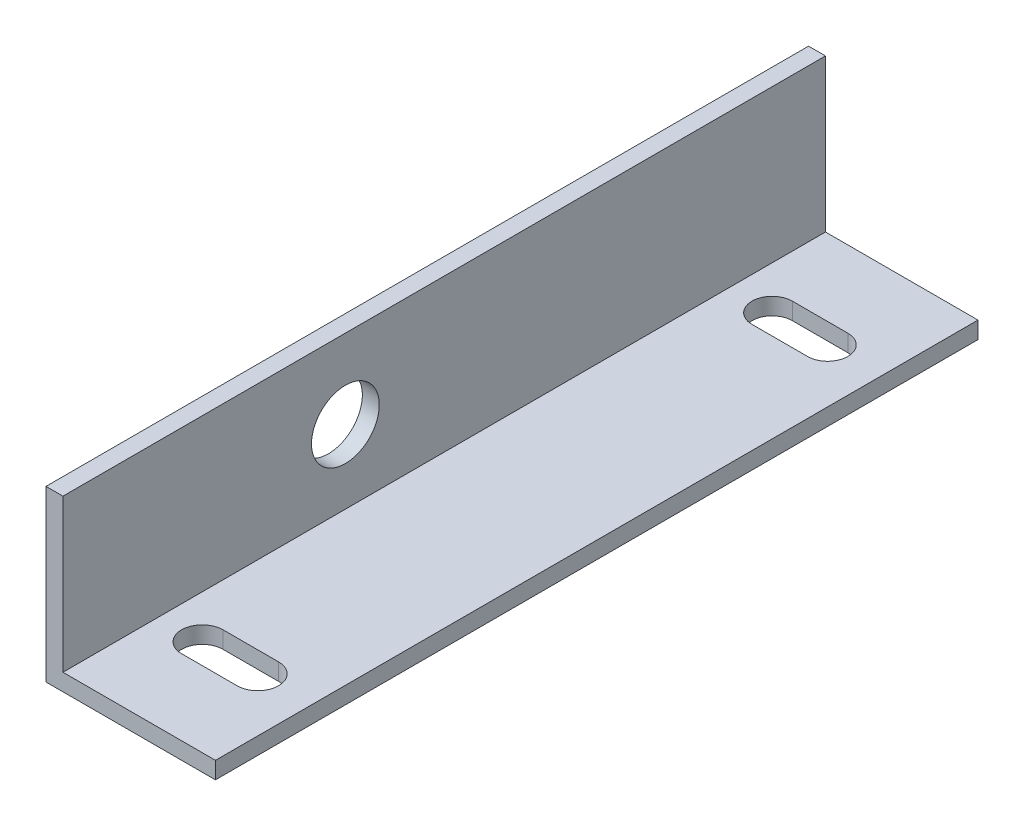
SolidWorks part; units mm, degrees
ref_plane "Front Plane" through (0, 0, 0) normal (0, 0, 1) x (1, 0, 0)
ref_plane "Top Plane" through (0, 0, 0) normal (0, 1, 0) x (1, 0, 0)
ref_plane "Right Plane" through (0, 0, 0) normal (1, 0, 0) x (0, 0, -1)
sketch "Sketch1" plane through (0, 0, 0) normal (0, 0, 1) x (1, 0, 0)
  line L0 (0, 0) -> (0, 30)
  line L1 (0, 0) -> (30, 0)
  line L2 (3, 3) -> (30, 3)
  line L3 (3, 3) -> (3, 30)
  line L4 (0, 30) -> (3, 30)
  line L5 (30, 3) -> (30, 0)
  dimension "D1" = 30
  dimension "D2" = 30
  dimension "D3" = 3
extrude "Boss-Extrude1" add sketch "Sketch1" along normal blind 135
sketch "Sketch2" plane through (0, 3, 0) normal (0, 1, 0) x (1, 0, 0)
  line L0 (10.659, -17.1008) -> (20.4946, -17.1008) construction
  line L1 (10.659, -13.5319) -> (20.4946, -13.5319)
  line L2 (10.659, -20.6697) -> (20.4946, -20.6697)
  line L3 (10.659, -117.9846) -> (20.4946, -117.9846) construction
  line L4 (10.659, -114.3178) -> (20.4946, -114.3178)
  line L5 (10.659, -121.6515) -> (20.4946, -121.6515)
  arc A0 (10.659, -13.5319) -> (10.659, -20.6697) centre (10.659, -17.1008) ccw
  arc A1 (20.4946, -20.6697) -> (20.4946, -13.5319) centre (20.4946, -17.1008) ccw
  arc A2 (10.659, -114.3178) -> (10.659, -121.6515) centre (10.659, -117.9846) ccw
  arc A3 (20.4946, -121.6515) -> (20.4946, -114.3178) centre (20.4946, -117.9846) ccw
  point P2 (15.5768, -17.1008)
  point P7 (15.5768, -117.9846)
extrude "Cut-Extrude1" cut sketch "Sketch2" against normal blind 160
sketch "Sketch3" plane through (0, 0, 0) normal (-1, 0, 0) x (0, 0, 1)
  line L0 (135, 30) -> (135, 0) construction
  line L1 (135, 0) -> (0, 0) construction
  circle A0 centre (85, 16) radius 6
  dimension "D1" = 12
  dimension "D2" = 50
  dimension "D3" = 16
extrude "Cut-Extrude2" cut sketch "Sketch3" against normal blind 10
